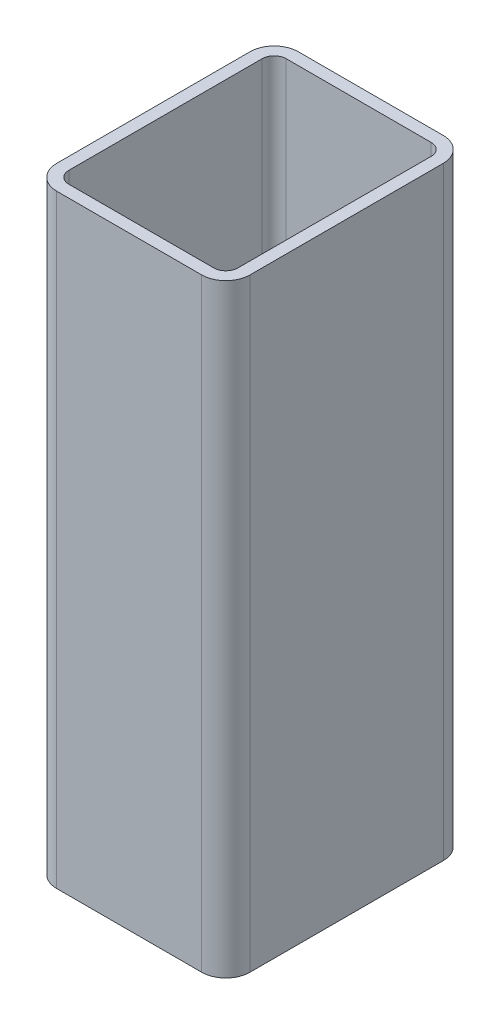
from build123d import *

# Parameters (mm, degrees)
GB_T_6728_2002_RECTANGULAR_HOLLOW_SECTIO_DEPTH = 250


with BuildPart() as part:
    # Sketch12 → Gb／t 6728—2002 rectangular hollow section 100X80X5(1) (new body)
    with BuildSketch(Plane(origin=(0, 0, 0), x_dir=(-1, 0, 0), z_dir=(0, 1, 0))):
        with BuildLine():
            Line((-30, -50), (30, -50))
            ThreePointArc((30, -50), (37.071067812, -47.071067812), (40, -40))
            Line((40, -40), (40, 40))
            ThreePointArc((40, 40), (37.071067812, 47.071067812), (30, 50))
            Line((30, 50), (-30, 50))
            ThreePointArc((-30, 50), (-37.071067812, 47.071067812), (-40, 40))
            Line((-40, 40), (-40, -40))
            ThreePointArc((-40, -40), (-37.071067812, -47.071067812), (-30, -50))
        make_face()
        with BuildLine():
            Line((-30, -45), (30, -45))
            ThreePointArc((30, -45), (33.535533906, -43.535533906), (35, -40))
            Line((35, -40), (35, 40))
            ThreePointArc((35, 40), (33.535533906, 43.535533906), (30, 45))
            Line((30, 45), (-30, 45))
            ThreePointArc((-30, 45), (-33.535533906, 43.535533906), (-35, 40))
            Line((-35, 40), (-35, -40))
            ThreePointArc((-35, -40), (-33.535533906, -43.535533906), (-30, -45))
        make_face(mode=Mode.SUBTRACT)
    extrude(amount=GB_T_6728_2002_RECTANGULAR_HOLLOW_SECTIO_DEPTH)


solid = part.part
